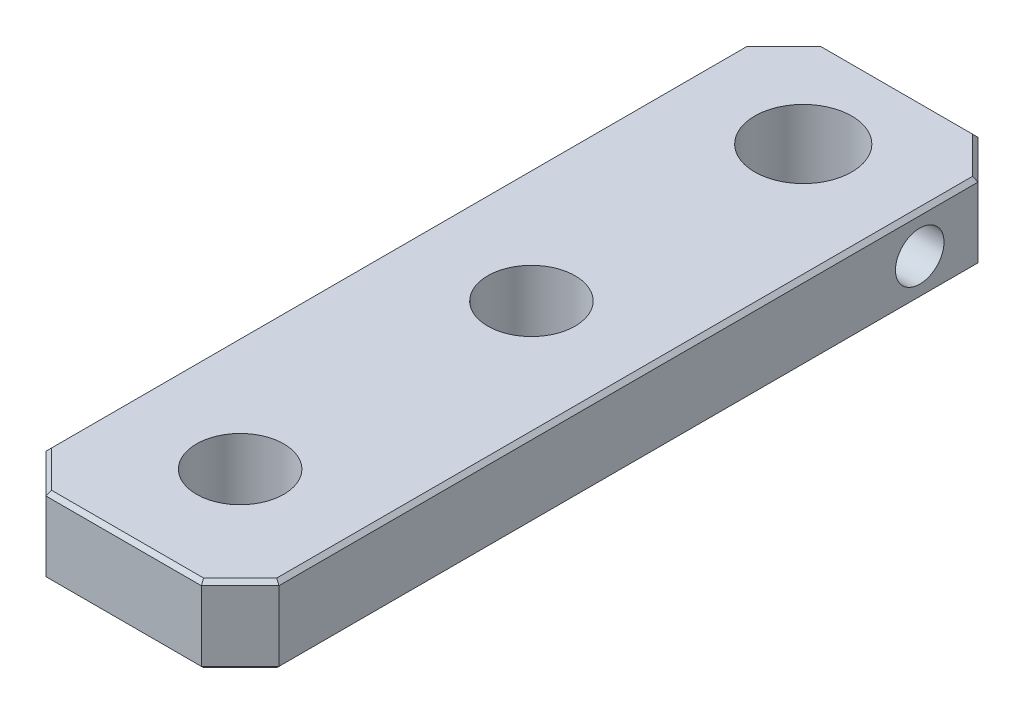
from build123d import *

# Parameters (mm, degrees)
SKETCH1_W                  = 12
SKETCH1_H                  = 40
BOSS_EXTRUDE1_DEPTH        = 2
CHAMFER1_SIZE              = 2
M6_TAPPED_HOLE1_D          = 5
F_4_5_4_5_DIAMETER_HOLE1_D = 4.5
M3_TAPPED_HOLE1_REACH      = 25.409
M3_TAPPED_HOLE1_BORE_R     = 1.25
CHAMFER2_SIZE              = 0.2


with BuildPart() as part:
    # Sketch1 → Boss-Extrude1 (new, symmetric)
    with BuildSketch(Plane(origin=(0, 0, 0), x_dir=(1, 0, 0), z_dir=(0, 1, 0))):
        Rectangle(SKETCH1_W, SKETCH1_H)
    extrude(amount=BOSS_EXTRUDE1_DEPTH, both=True)

    # Chamfer1
    chamfer1_edges = [part.edges().sort_by_distance(p)[0] for p in [
        (6, 0, 20),
        (-6, 0, 20),
        (-6, 0, -20),
        (6, 0, -20),
    ]]
    chamfer(chamfer1_edges, length=CHAMFER1_SIZE)

    # M6 Tapped Hole1 (through all)
    with Locations(Plane(origin=(0, 2, 0), x_dir=(1, 0, 0), z_dir=(0, 1, 0))):
        with Locations((0, 15)):
            Hole(M6_TAPPED_HOLE1_D / 2)

    # Ø4.5 (4.5) Diameter Hole1 (through all)
    with Locations(Plane(origin=(0, 2, 0), x_dir=(1, 0, 0), z_dir=(0, 1, 0))):
        with Locations((0, 1), (0, -14)):
            Hole(F_4_5_4_5_DIAMETER_HOLE1_D / 2)

    # M3 Tapped Hole1 bore → M3 Tapped Hole1 (cut, up to next)
    with BuildSketch(Plane(origin=(6, 0, 0), x_dir=(0, 0, -1), z_dir=(1, 0, 0)), mode=Mode.PRIVATE) as m3_tapped_hole1_sk1:
        with Locations((15, 0)):
            Circle(M3_TAPPED_HOLE1_BORE_R)
    m3_tapped_hole1_tool1 = extrude(m3_tapped_hole1_sk1.sketch, amount=-M3_TAPPED_HOLE1_REACH, mode=Mode.PRIVATE) & part.part
    add(m3_tapped_hole1_tool1.solids().sort_by_distance((6, 0, -15))[0], mode=Mode.SUBTRACT)

    # Chamfer2
    chamfer2_edges = [part.edges().sort_by_distance(p)[0] for p in [
        (-6, -2, 0),
        (-6, 2, 0),
        (6, -2, 0),
        (0, -2, 20),
        (0, -2, -20),
        (-5, -2, 19),
        (5, -2, 19),
        (5, -2, -19),
        (-5, -2, -19),
        (0, 2, -20),
        (6, 2, 0),
        (0, 2, 20),
        (-5, 2, 19),
        (5, 2, 19),
        (5, 2, -19),
        (-5, 2, -19),
    ]]
    chamfer(chamfer2_edges, length=CHAMFER2_SIZE)


solid = part.part
